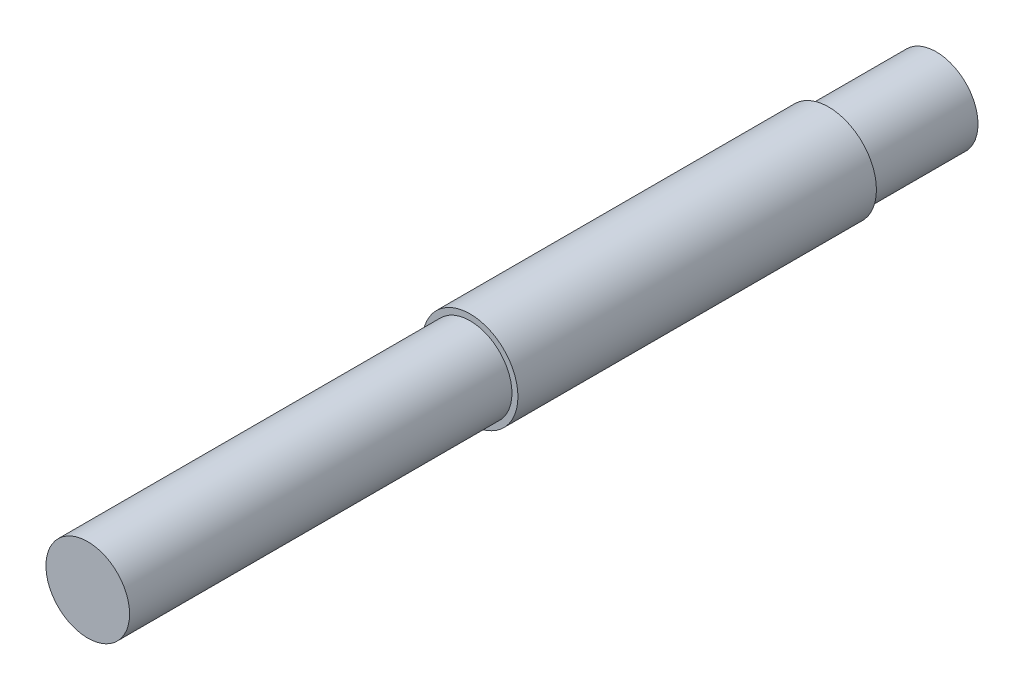
from build123d import *

# Parameters (mm, degrees)
SKETCH_1_R      = 20
EXTRUDE_1_DEPTH = 150
SKETCH_2_R      = 17.5
EXTRUDE_2_DEPTH = 160
EXTRUDE_START   = 45
SKETCH_3_R      = 17.5
EXTRUDE_3_DEPTH = 45


with BuildPart() as part:
    # 草图1 → 凸台-拉伸1 (new body)
    with BuildSketch(Plane.XY):
        Circle(SKETCH_1_R)
    extrude(amount=EXTRUDE_1_DEPTH)

    # 草图2 → 凸台-拉伸2 (add)
    with BuildSketch(Plane.XY.offset(150)):
        Circle(SKETCH_2_R)
    extrude(amount=EXTRUDE_2_DEPTH)

    # 草图3 → 凸台-拉伸3 (add)
    with BuildSketch(Plane(origin=(0, 0, 0), x_dir=(-1, 0, 0), z_dir=(0, 0, -1)).offset(EXTRUDE_START)):
        with Locations(Location((0, 0, 0), (0, 0, 180))):
            Circle(SKETCH_3_R)
    extrude(amount=-EXTRUDE_3_DEPTH)


solid = part.part
